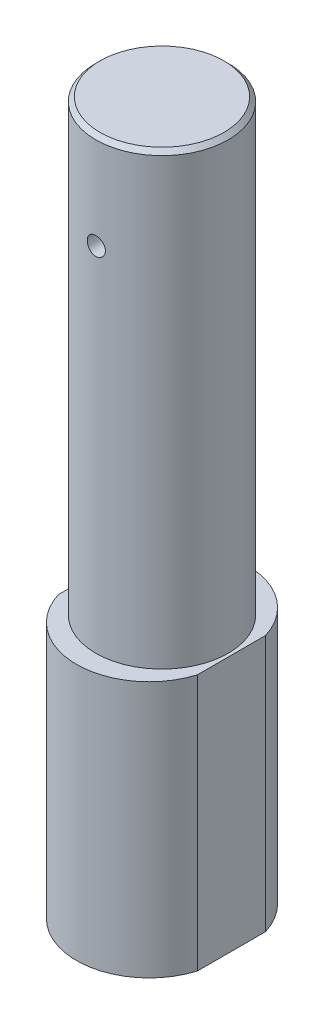
from build123d import *

# Parameters (mm, degrees)
EXTRUDE_1_DEPTH         = 120
SKETCH_2_R              = 31
EXTRUDE_2_DEPTH         = 210
HOLE_WIZARD_M10_1_D     = 8.5
HOLE_WIZARD_M10_1_DEPTH = 27.5
HOLE_WIZARD_M10_1_TIP   = 2.553657631
CHAMFER_1_SIZE          = 2


with BuildPart() as part:
    # 草图1 → 凸台-拉伸1 (new body)
    with BuildSketch(Plane(origin=(0, 0, 0), x_dir=(1, 0, 0), z_dir=(0, 1, 0))):
        with BuildLine():
            Line((32.5, -15.987492178), (32.5, 15.987492178))
            ThreePointArc((32.5, 15.987492178), (0, 40), (-32.5, 15.987492178))
            Line((-32.5, 15.987492178), (-32.5, -15.987492178))
            ThreePointArc((-32.5, -15.987492178), (0, -40), (32.5, -15.987492178))
        make_face()
    extrude(amount=EXTRUDE_1_DEPTH)

    # 草图2 → 凸台-拉伸2 (add)
    with BuildSketch(Plane(origin=(0, 120, 0), x_dir=(1, 0, 0), z_dir=(0, 1, 0))):
        with Locations(Location((0, 0, 0), (0, 0, 270))):
            Circle(SKETCH_2_R)
    extrude(amount=EXTRUDE_2_DEPTH)

    # M10 螺纹孔1
    with Locations(Plane.XY.offset(31)):
        with Locations((0, 285)):
            Hole(HOLE_WIZARD_M10_1_D / 2, depth=HOLE_WIZARD_M10_1_DEPTH)
            with Locations((0, 0, -(HOLE_WIZARD_M10_1_DEPTH + HOLE_WIZARD_M10_1_TIP / 2))):  # 118° drill point
                Cone(0, HOLE_WIZARD_M10_1_D / 2, HOLE_WIZARD_M10_1_TIP, mode=Mode.SUBTRACT)

    # 倒角1
    chamfer_1_edges = [part.edges().sort_by_distance(p)[0] for p in [
        (0, 330, -31),
    ]]
    chamfer(chamfer_1_edges, length=CHAMFER_1_SIZE)


solid = part.part
